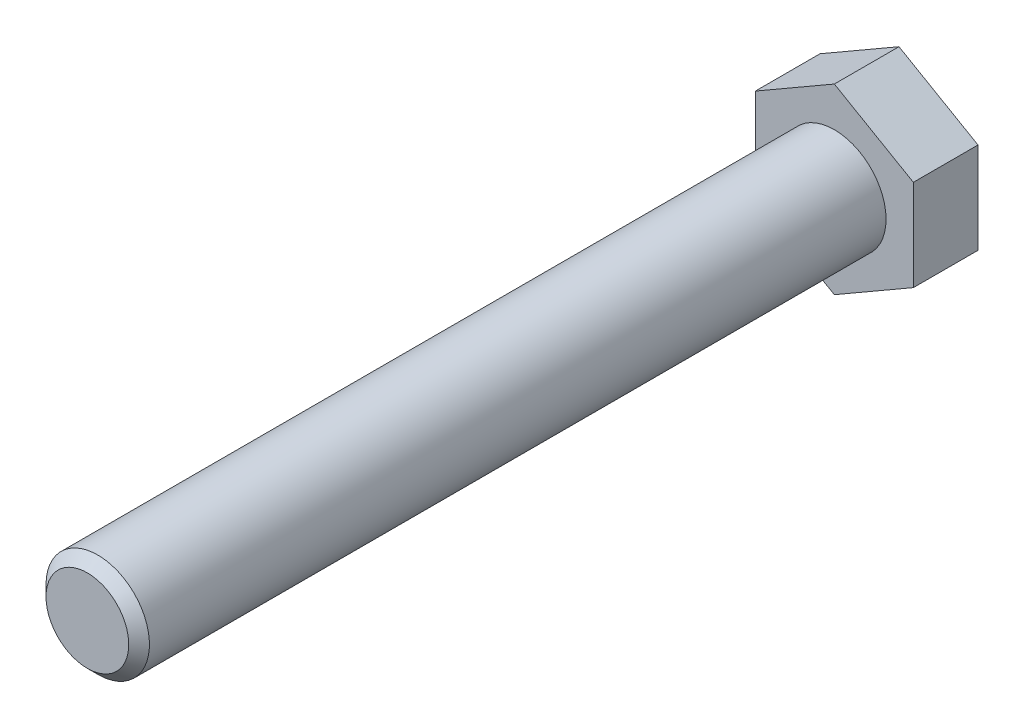
from build123d import *

# Parameters (mm, degrees)
BOSS_EXTRUDE1_DEPTH = 22.5
SKETCH3_R           = 18
BOSS_EXTRUDE2_DEPTH = 260
CHAMFER1_SIZE       = 3.6


with BuildPart() as part:
    # Sketch1 → Boss-Extrude1 (new body)
    with BuildSketch(Plane.XY):
        Polygon((27.5, 15.877132403), (0, 31.754264805), (-27.5, 15.877132403), (-27.5, -15.877132403), (0, -31.754264805), (27.5, -15.877132403), align=None)
    extrude(amount=BOSS_EXTRUDE1_DEPTH)

    # Sketch3 → Boss-Extrude2 (add)
    with BuildSketch(Plane.XY.offset(22.5)):
        Circle(SKETCH3_R)
    extrude(amount=BOSS_EXTRUDE2_DEPTH)

    # Chamfer1
    chamfer1_edges = [part.edges().sort_by_distance(p)[0] for p in [
        (-18, 0, 282.5),
    ]]
    chamfer(chamfer1_edges, length=CHAMFER1_SIZE)


solid = part.part
